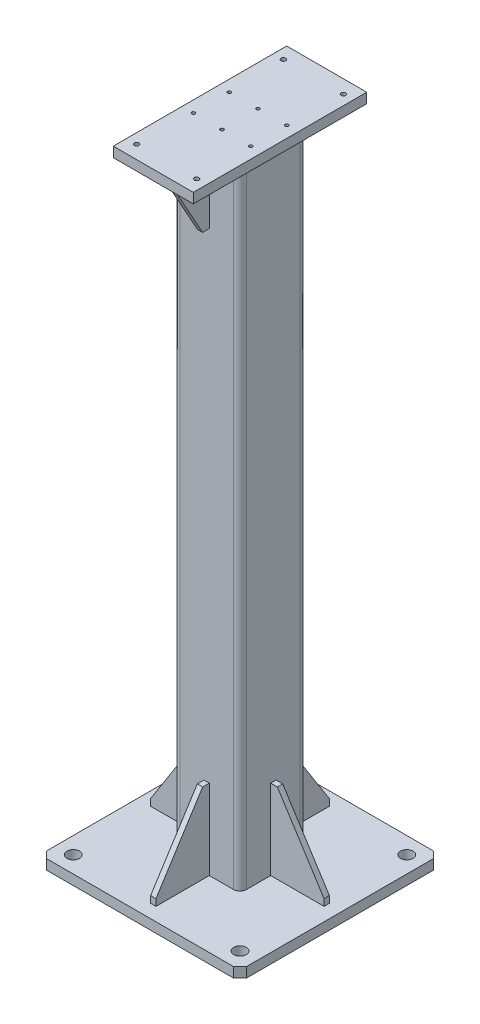
from build123d import *

# Parameters (mm, degrees)
F_100_X_100_X_5_1_DEPTH          = 940
SKETCH_4_W                       = 300
SKETCH_4_H                       = 300
EXTRUDE_1_DEPTH                  = 15
SKETCH_5_W                       = 120
SKETCH_5_H                       = 260
EXTRUDE_2_DEPTH                  = 15
GUSSET_1_THICKNESS               = 8
GUSSET_2_THICKNESS               = 8
GUSSET_3_THICKNESS               = 8
GUSSET_4_THICKNESS               = 8
GUSSET_5_THICKNESS               = 8
GUSSET_6_THICKNESS               = 8
HOLE_WIZARD_19_0_19_1_AT_2_COUNT = 2
HOLE_WIZARD_19_0_19_1_AT_2_PITCH = 250
HOLE_WIZARD_19_0_19_1_AT_3_COUNT = 2
HOLE_WIZARD_19_0_19_1_AT_3_PITCH = 353.553390593
HOLE_WIZARD_19_0_19_1_AT_4_COUNT = 2
HOLE_WIZARD_19_0_19_1_AT_4_PITCH = 250
HOLE_WIZARD_M8_1_AT_2_COUNT      = 2
HOLE_WIZARD_M8_1_AT_2_PITCH      = 90
HOLE_WIZARD_M8_1_AT_3_COUNT      = 2
HOLE_WIZARD_M8_1_AT_3_PITCH      = 237.69728648
HOLE_WIZARD_M8_1_AT_4_COUNT      = 2
HOLE_WIZARD_M8_1_AT_4_PITCH      = 220
CHAMFER_1_SIZE                   = 10
HOLE_WIZARD_M6_1_AT_2_COUNT      = 2
HOLE_WIZARD_M6_1_AT_2_PITCH      = 43


with BuildPart() as part:
    # Sketch12 → 方形管 100 X 100 X 5(1) (new body)
    with BuildSketch(Plane(origin=(0, 0, 0), x_dir=(-1, 0, 0), z_dir=(0, 1, 0))):
        with BuildLine():
            Line((-40, -50), (40, -50))
            ThreePointArc((40, -50), (47.071067812, -47.071067812), (50, -40))
            Line((50, -40), (50, 40))
            ThreePointArc((50, 40), (47.071067812, 47.071067812), (40, 50))
            Line((40, 50), (-40, 50))
            ThreePointArc((-40, 50), (-47.071067812, 47.071067812), (-50, 40))
            Line((-50, 40), (-50, -40))
            ThreePointArc((-50, -40), (-47.071067812, -47.071067812), (-40, -50))
        make_face()
        with BuildLine():
            Line((-40, -45), (40, -45))
            ThreePointArc((40, -45), (43.535533906, -43.535533906), (45, -40))
            Line((45, -40), (45, 40))
            ThreePointArc((45, 40), (43.535533906, 43.535533906), (40, 45))
            Line((40, 45), (-40, 45))
            ThreePointArc((-40, 45), (-43.535533906, 43.535533906), (-45, 40))
            Line((-45, 40), (-45, -40))
            ThreePointArc((-45, -40), (-43.535533906, -43.535533906), (-40, -45))
        make_face(mode=Mode.SUBTRACT)
    extrude(amount=F_100_X_100_X_5_1_DEPTH)


with BuildPart() as body_2:
    # 草图4 → 凸台-拉伸1 (new body)
    with BuildSketch(Plane.XZ):
        Rectangle(SKETCH_4_W, SKETCH_4_H)
    extrude(amount=EXTRUDE_1_DEPTH)

    # 草图13 → Ø19.0 (19) 直径孔1 (revolve, cut)
    with BuildSketch(Plane(origin=(125, 0, 125), x_dir=(0, 0, 1), z_dir=(1, 0, 0))):
        Polygon((0, 0), (0, 33.208175881), (9.5, 27.5), (9.5, 0), align=None)
    hole_wizard_19_0_19_1 = revolve(axis=Axis((125, 6.35, 125), (0, -1, 0)), mode=Mode.SUBTRACT)

    # Ø19.0 (19) 直径孔1 at 2: Ø19.0 (19) 直径孔1 ×2
    with Locations(*[(0, 0, -i * HOLE_WIZARD_19_0_19_1_AT_2_PITCH) for i in range(1, HOLE_WIZARD_19_0_19_1_AT_2_COUNT)]):
        add(hole_wizard_19_0_19_1, mode=Mode.SUBTRACT)

    # Ø19.0 (19) 直径孔1 at 3: Ø19.0 (19) 直径孔1 ×2
    with Locations(*[Vector(-0.7071067811865476, 0, -0.7071067811865476) * (i * HOLE_WIZARD_19_0_19_1_AT_3_PITCH) for i in range(1, HOLE_WIZARD_19_0_19_1_AT_3_COUNT)]):
        add(hole_wizard_19_0_19_1, mode=Mode.SUBTRACT)

    # Ø19.0 (19) 直径孔1 at 4: Ø19.0 (19) 直径孔1 ×2
    with Locations(*[(-i * HOLE_WIZARD_19_0_19_1_AT_4_PITCH, 0, 0) for i in range(1, HOLE_WIZARD_19_0_19_1_AT_4_COUNT)]):
        add(hole_wizard_19_0_19_1, mode=Mode.SUBTRACT)

    # 倒角1
    chamfer_1_edges = [body_2.edges().sort_by_distance(p)[0] for p in [
        (150, -7.5, -150),
        (-150, -7.5, -150),
        (-150, -7.5, 150),
        (150, -7.5, 150),
    ]]
    chamfer(chamfer_1_edges, length=CHAMFER_1_SIZE)


with BuildPart() as body_3:
    # 草图5 → 凸台-拉伸2 (new body)
    with BuildSketch(Plane(origin=(0, 940, 0), x_dir=(1, 0, 0), z_dir=(0, 1, 0))):
        Rectangle(SKETCH_5_W, SKETCH_5_H)
    extrude(amount=EXTRUDE_2_DEPTH)

    # 草图15 → M8 螺纹孔1 (revolve, cut)
    with BuildSketch(Plane(origin=(45, 940, 110), x_dir=(0, 0, -1), z_dir=(1, 0, 0))):
        Polygon((0, 0), (0, 21.792926105), (3.4, 19.75), (3.4, 0), align=None)
    hole_wizard_m8_1 = revolve(axis=Axis((45, 933.65, 110), (0, 1, 0)), mode=Mode.SUBTRACT)

    # M8 螺纹孔1 at 2: M8 螺纹孔1 ×2
    with Locations(*[(-i * HOLE_WIZARD_M8_1_AT_2_PITCH, 0, 0) for i in range(1, HOLE_WIZARD_M8_1_AT_2_COUNT)]):
        add(hole_wizard_m8_1, mode=Mode.SUBTRACT)

    # M8 螺纹孔1 at 3: M8 螺纹孔1 ×2
    with Locations(*[Vector(-0.37863284572050415, 0, -0.9255469562056767) * (i * HOLE_WIZARD_M8_1_AT_3_PITCH) for i in range(1, HOLE_WIZARD_M8_1_AT_3_COUNT)]):
        add(hole_wizard_m8_1, mode=Mode.SUBTRACT)

    # M8 螺纹孔1 at 4: M8 螺纹孔1 ×2
    with Locations(*[(0, 0, -i * HOLE_WIZARD_M8_1_AT_4_PITCH) for i in range(1, HOLE_WIZARD_M8_1_AT_4_COUNT)]):
        add(hole_wizard_m8_1, mode=Mode.SUBTRACT)

    # 草图19 → M6 螺纹孔1 (revolve, cut)
    with BuildSketch(Plane(origin=(-43, 955, -27), x_dir=(0, 0, 1), z_dir=(1, 0, 0))):
        Polygon((0, 0), (0, 16.502151548), (2.5, 15), (2.5, 0), align=None)
    hole_wizard_m6_1 = revolve(axis=Axis((-43, 961.35, -27), (0, -1, 0)), mode=Mode.SUBTRACT)

    # M6 螺纹孔1 at 2: M6 螺纹孔1 ×2
    with Locations(*[(i * HOLE_WIZARD_M6_1_AT_2_PITCH, 0, 0) for i in range(1, HOLE_WIZARD_M6_1_AT_2_COUNT)]):
        add(hole_wizard_m6_1, mode=Mode.SUBTRACT)

    # 草图20 → M6 螺纹孔2 (revolve, cut)
    with BuildSketch(Plane(origin=(43, 955, -27), x_dir=(0, 0, 1), z_dir=(1, 0, 0))):
        Polygon((0, 0), (0, 16.502151548), (2.5, 15), (2.5, 0), align=None)
    hole_wizard_m6_2 = revolve(axis=Axis((43, 961.35, -27), (0, -1, 0)), mode=Mode.SUBTRACT)

    # 镜向1: M6 螺纹孔1, M6 螺纹孔2 across plane
    add(hole_wizard_m6_1.mirror(Plane.XY), mode=Mode.SUBTRACT)
    add(hole_wizard_m6_2.mirror(Plane.XY), mode=Mode.SUBTRACT)

    # 镜向1 copy 1 sketch → 镜向1 copy 1 (revolve, cut)
    with BuildSketch(Plane(origin=(0, 955, 27), x_dir=(0, 0, -1), z_dir=(1, 0, 0))):
        Polygon((0, 0), (0, -16.502151548), (2.5, -15), (2.5, 0), align=None)
    revolve(axis=Axis((0, 961.35, 27), (0, 1, 0)), mode=Mode.SUBTRACT)


with BuildPart() as body_4:
    # Gusset 1: a gusset: a plate 8.0 thick in the corner of two members, its outline drawn in place
    gusset_1_outline = Wire([Line((50, 0, -4), (50, 120, -4)), Line((50, 120, -4), (60, 120, -4)), Line((60, 120, -4), (130, 10, -4)), Line((130, 10, -4), (130, 0, -4)), Line((130, 0, -4), (50, 0, -4))])
    add(extrude(Face(gusset_1_outline), amount=GUSSET_1_THICKNESS, dir=(0, 0, 1)))


with BuildPart() as body_5:
    # Gusset 2: a gusset: a plate 8.0 thick in the corner of two members, its outline drawn in place
    gusset_2_outline = Wire([Line((-4, 0, -50), (-4, 120, -50)), Line((-4, 120, -50), (-4, 120, -60)), Line((-4, 120, -60), (-4, 10, -130)), Line((-4, 10, -130), (-4, 0, -130)), Line((-4, 0, -130), (-4, 0, -50))])
    add(extrude(Face(gusset_2_outline), amount=GUSSET_2_THICKNESS, dir=(1, 0, 0)))


with BuildPart() as body_6:
    # Gusset 3: a gusset: a plate 8.0 thick in the corner of two members, its outline drawn in place
    gusset_3_outline = Wire([Line((-50, 0, 4), (-50, 120, 4)), Line((-50, 120, 4), (-60, 120, 4)), Line((-60, 120, 4), (-130, 10, 4)), Line((-130, 10, 4), (-130, 0, 4)), Line((-130, 0, 4), (-50, 0, 4))])
    add(extrude(Face(gusset_3_outline), amount=GUSSET_3_THICKNESS, dir=(0, 0, -1)))


with BuildPart() as body_7:
    # Gusset 4: a gusset: a plate 8.0 thick in the corner of two members, its outline drawn in place
    gusset_4_outline = Wire([Line((4, 0, 50), (4, 120, 50)), Line((4, 120, 50), (4, 120, 60)), Line((4, 120, 60), (4, 10, 130)), Line((4, 10, 130), (4, 0, 130)), Line((4, 0, 130), (4, 0, 50))])
    add(extrude(Face(gusset_4_outline), amount=GUSSET_4_THICKNESS, dir=(-1, 0, 0)))


with BuildPart() as body_8:
    # Gusset 5: a gusset: a plate 8.0 thick in the corner of two members, its outline drawn in place
    gusset_5_outline = Wire([Line((4, 940, -50), (4, 840, -50)), Line((4, 840, -50), (4, 840, -60)), Line((4, 840, -60), (4, 930, -110)), Line((4, 930, -110), (4, 940, -110)), Line((4, 940, -110), (4, 940, -50))])
    add(extrude(Face(gusset_5_outline), amount=GUSSET_5_THICKNESS, dir=(-1, 0, 0)))


with BuildPart() as body_9:
    # Gusset 6: a gusset: a plate 8.0 thick in the corner of two members, its outline drawn in place
    gusset_6_outline = Wire([Line((-4, 940, 50), (-4, 840, 50)), Line((-4, 840, 50), (-4, 840, 60)), Line((-4, 840, 60), (-4, 930, 110)), Line((-4, 930, 110), (-4, 940, 110)), Line((-4, 940, 110), (-4, 940, 50))])
    add(extrude(Face(gusset_6_outline), amount=GUSSET_6_THICKNESS, dir=(1, 0, 0)))


solid = Compound([part.part, body_2.part, body_3.part, body_4.part, body_5.part, body_6.part, body_7.part, body_8.part, body_9.part])
